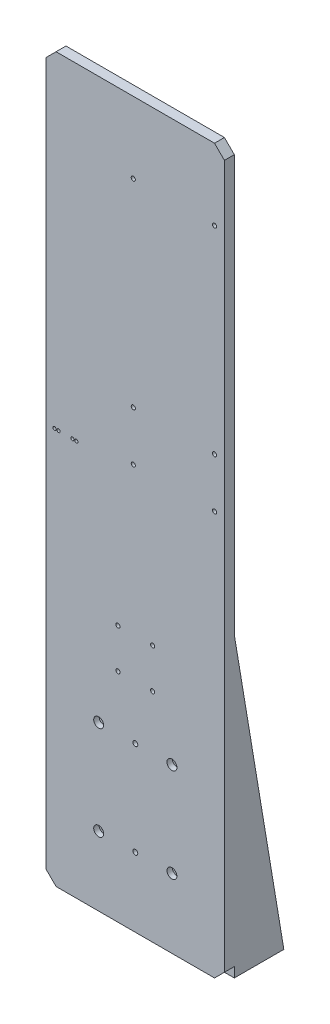
from build123d import *

# Parameters (mm, degrees)
SKETCH_1_W                   = 180
SKETCH_1_H                   = 730
EXTRUDE_1_DEPTH              = 10
HOLE_WIZARD_M5_1_D           = 5.5
HOLE_WIZARD_M5_1_CBORE_D     = 10
HOLE_WIZARD_M5_1_CBORE_DEPTH = 5.4
MM_0_D                       = 5
CHAMFER_1_SIZE               = 10
HOLE_WIZARD_M5_2_D           = 4.2
HOLE_WIZARD_M5_3_D           = 4.2
HOLE_WIZARD_M4_1_D           = 3.3
EXTRUDE_2_DEPTH              = 10


with BuildPart() as part:
    # 草图1 → 凸台-拉伸1 (new body)
    with BuildSketch(Plane.XY):
        Rectangle(SKETCH_1_W, SKETCH_1_H)
    extrude(amount=EXTRUDE_1_DEPTH)

    # M5 六角凹头螺钉的柱形沉头孔1 (through all)
    with Locations(Plane.XY.offset(10)):
        with Locations((-37, -200), (37, -200), (-37, -295), (37, -295)):
            CounterBoreHole(HOLE_WIZARD_M5_1_D / 2, HOLE_WIZARD_M5_1_CBORE_D / 2, HOLE_WIZARD_M5_1_CBORE_DEPTH)

    # 大小mm 暗销孔0 (through all)
    with Locations(Plane.XY.offset(10)):
        with Locations((0, -200), (0, -295)):
            Hole(MM_0_D / 2)

    # 倒角1
    chamfer_1_edges = [part.edges().sort_by_distance(p)[0] for p in [
        (90, -365, 5),
        (-90, -365, 5),
        (-90, 365, 5),
        (90, 365, 5),
    ]]
    chamfer(chamfer_1_edges, length=CHAMFER_1_SIZE)

    # M5 螺纹孔2 (through all)
    with Locations(Plane.XY.offset(10)):
        with Locations((80, 293), (-2, 293), (80, 93), (80, 43), (-2, 43), (-2, 93)):
            Hole(HOLE_WIZARD_M5_2_D / 2)

    # M5 螺纹孔3 (through all)
    with Locations(Plane(origin=(0, 0, 0), x_dir=(-1, 0, 0), z_dir=(0, 0, -1))):
        with Locations((-17.5, -105.532443279), (-17.5, -145.532443279), (17.5, -105.532443279), (17.5, -145.532443279)):
            Hole(HOLE_WIZARD_M5_3_D / 2)

    # M4 螺纹孔1 (through all)
    with Locations(Plane.XY.offset(10)):
        with Locations((-81.499026454, 34.792936996), (-59.499927509, 34.792936996), (-77.499026454, 34.792936996), (-63.499026454, 34.792936996)):
            Hole(HOLE_WIZARD_M4_1_D / 2)

    # 草图12 → 凸台-拉伸2 (add)
    with BuildSketch(Plane.ZY.offset(90)):
        Polygon((0, -65), (-50, -365), (0, -365), align=None)
    extrude_2 = extrude(amount=-EXTRUDE_2_DEPTH)

    # 镜向1: 凸台-拉伸2 across plane
    add(extrude_2.mirror(Plane(origin=(0, 0, 0), x_dir=(0, 0, 1), z_dir=(1, 0, 0))))


solid = part.part
